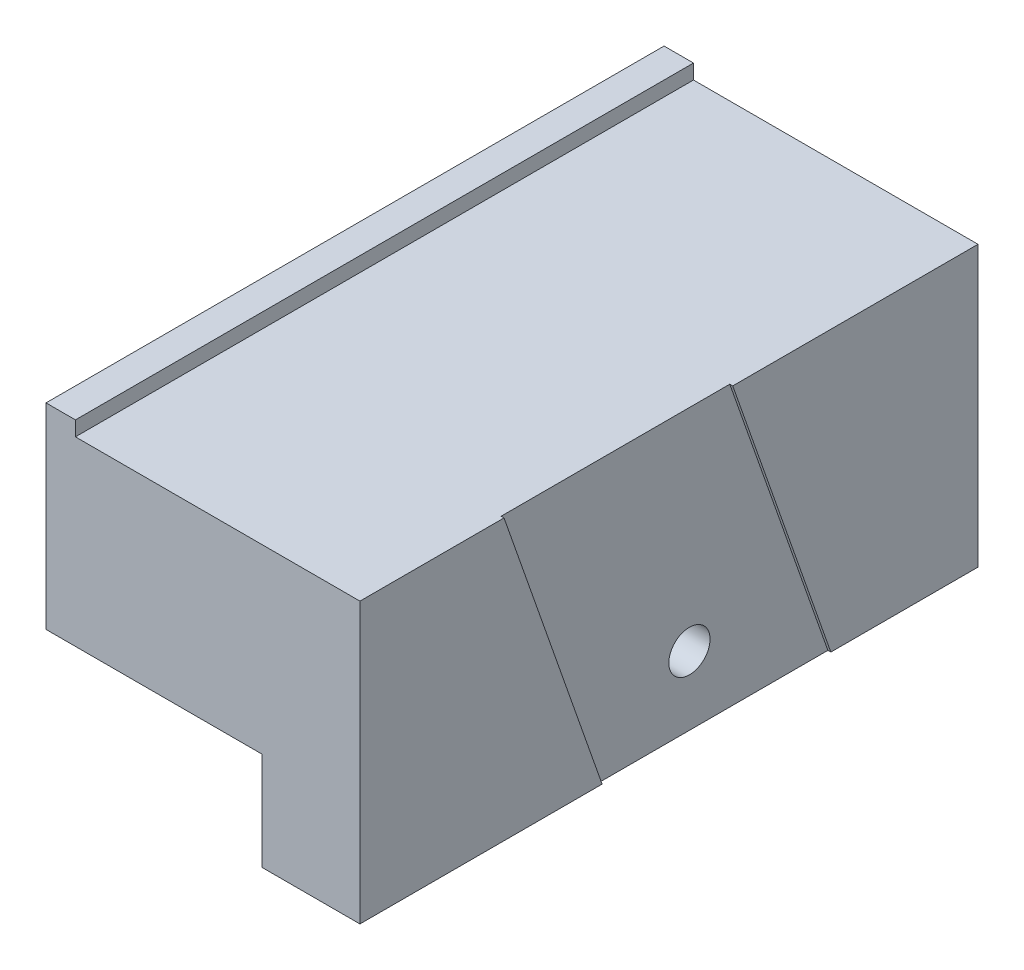
from build123d import *

# Parameters (mm, degrees)
EXTRUDE_1_DEPTH     = 31.5
SKETCH_2_W          = 29
SKETCH_2_H          = 63
CUT_EXTRUDE_1_DEPTH = 1.5
CUT_EXTRUDE_2_DEPTH = 0.3
HOLE_WIZARD_M5_1_D  = 4.2


with BuildPart() as part:
    # 草图1 → 凸台-拉伸1 (new, symmetric)
    with BuildSketch(Plane.XY):
        Polygon((0, 0), (32, 0), (32, -30), (22, -30), (22, -20), (0, -20), align=None)
    extrude(amount=EXTRUDE_1_DEPTH, both=True)

    # 草图2 → 切除-拉伸1 (cut)
    with BuildSketch(Plane(origin=(0, 0, 0), x_dir=(1, 0, 0), z_dir=(0, 1, 0))):
        with Locations((17.5, 0)):
            Rectangle(SKETCH_2_W, SKETCH_2_H)
    extrude(amount=-CUT_EXTRUDE_1_DEPTH, mode=Mode.SUBTRACT)

    # 草图3 → 切除-拉伸2 (cut)
    with BuildSketch(Plane(origin=(32, 0, 0), x_dir=(0, 0, -1), z_dir=(1, 0, 0))):
        Polygon((-16.814964409, -1.5), (-6.814964409, -30), (16.5, -30), (6.5, -1.5), align=None)
    extrude(amount=-CUT_EXTRUDE_2_DEPTH, mode=Mode.SUBTRACT)

    # M5 螺纹孔1 (through all)
    with Locations(Plane(origin=(31.7, -23, -2.386377444), x_dir=(0, 0, 1), z_dir=(1, 0, 0))):
        with Locations((0, 0)):
            Hole(HOLE_WIZARD_M5_1_D / 2)


solid = part.part
